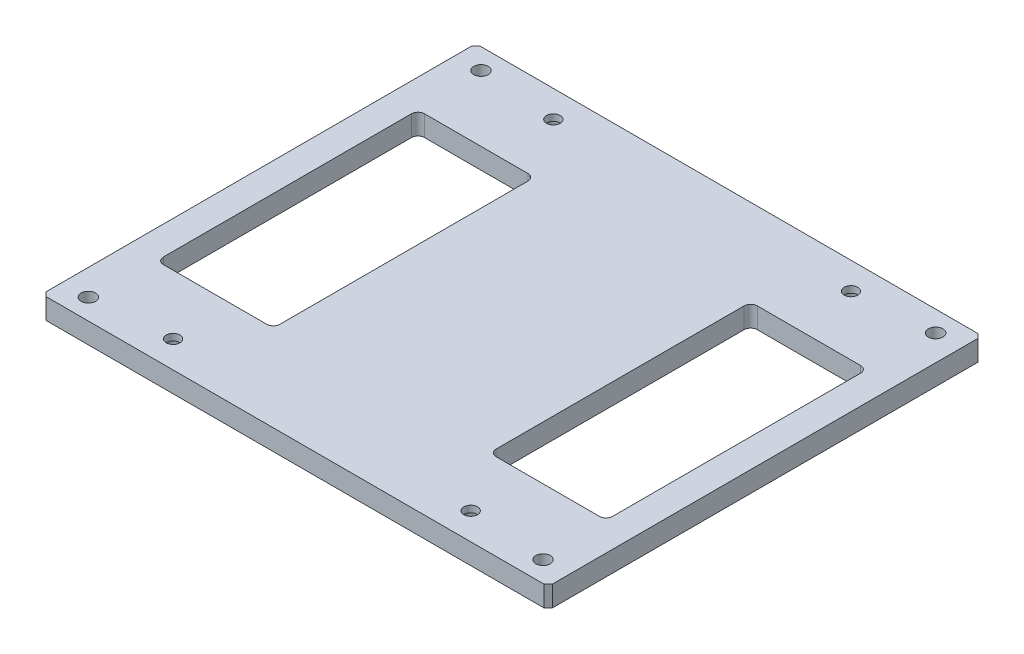
SolidWorks part; units mm, degrees
ref_plane "前视基准面" through (0, 0, 0) normal (0, 0, 1) x (1, 0, 0)
ref_plane "上视基准面" through (0, 0, 0) normal (0, 1, 0) x (1, 0, 0)
ref_plane "右视基准面" through (0, 0, 0) normal (1, 0, 0) x (0, 0, -1)
sketch "草图1" plane through (0, 0, 0) normal (0, 1, 0) x (1, 0, 0)
  line L1 (-122.5, -105) -> (122.5, -105)
  line L2 (-122.5, -105) -> (-122.5, 105)
  line L3 (-122.5, 105) -> (122.5, 105)
  line L4 (122.5, -105) -> (122.5, 105)
  line L5 (-122.5, -105) -> (122.5, 105) construction
  line L6 (-122.5, 105) -> (122.5, -105) construction
  point P0 (0, 0)
  dimension "D1" = 210
  dimension "D2" = 245
extrude "凸台-拉伸1" add sketch "草图1" along normal blind 10
sketch "草图3" plane through (0, 0, 0) normal (0, -1, 0) x (1, 0, 0)
  line L1 (-122.5, 105) -> (122.5, 105) construction
  circle A0 centre (72, 92) radius 3.5
  dimension "D1" = 7
  dimension "D2" = 72
  dimension "D3" = 13
chamfer "倒角1" distance 2 angle 45 4 edges at (-122.5, 5, 105) (-122.5, 5, -105) (122.5, 5, -105) (122.5, 5, 105)
hole_wizard "打孔尺寸(%根据)内六角圆柱头螺钉的类型1" positions "3D草图1" profile "草图4" counterbore size "M6" standard "GB" end condition up to next
sketch3d "3D草图1"
  point P0 (72, 0, 92)
  point P6 (0, 0, 0)
sketch "草图4" plane through (72, 0, 92) normal (1, 0, 0) x (0, 0, -1)
  line L0 (0, 0) -> (0, 10.001)
  line L1 (0, 10.001) -> (3.3, 10.001)
  line L3 (3.3, 10.001) -> (3.3, 6.8)
  line L4 (5.5, 6.8) -> (3.3, 6.8)
  line L5 (5.5, 6.8) -> (5.5, 0.025)
  line L6 (5.5, 0.025) -> (5.525, 0)
  line L7 (5.525, 0) -> (0, 0)
  line L8 (-5.5, 0.025) -> (-5.525, 0) construction
  line L11 (0, -6.35) -> (0, 107.95) construction
  dimension "通孔孔直径" = 6.6
  dimension "通孔孔深度" = 10.001
  dimension "柱形沉头孔直径" = 11
  dimension "柱形沉头孔深度" = 6.8
  dimension "近端锥形沉头孔直径" = 11.05
  dimension "近端锥形沉头孔角度" = 90
mirror "镜向1" about plane through (0, 0, 0) normal (1, 0, 0) of "打孔尺寸(%根据)内六角圆柱头螺钉的类型1"
mirror "镜向2" about plane through (0, 0, 0) normal (0, 0, 1) of "镜向1", "打孔尺寸(%根据)内六角圆柱头螺钉的类型1"
sketch "草图5" plane through (0, 10, 0) normal (0, 1, 0) x (1, 0, 0)
  line L0 (120.5, 105) -> (-120.5, 105) construction
  line L1 (-110, -95) -> (110, -95) construction
  line L2 (-110, -95) -> (-110, 95) construction
  line L3 (-110, 95) -> (110, 95) construction
  line L4 (110, -95) -> (110, 95) construction
  line L5 (-110, -95) -> (110, 95) construction
  line L6 (-110, 95) -> (110, -95) construction
  circle A0 centre (-110, 95) radius 3.5
  circle A1 centre (110, 95) radius 3.5
  circle A2 centre (110, -95) radius 3.5
  circle A3 centre (-110, -95) radius 3.5
  point P0 (0, 0)
  dimension "D3" = 7
  dimension "D1" = 10
  dimension "D2" = 110
extrude "切除-拉伸1" cut sketch "草图5" against normal up to next
sketch "草图6" plane through (0, 10, 0) normal (0, 1, 0) x (1, 0, 0)
  line L0 (105.5, -63.2) -> (55.5, -63.2) construction
  line L1 (108.7, 60) -> (108.7, -60) construction
  line L2 (55.5, 63.2) -> (105.5, 63.2) construction
  line L3 (52.3, -60) -> (52.3, 60) construction
  line L4 (105.5, -63.2) -> (55.5, -63.2)
  line L5 (108.7, 60) -> (108.7, -60)
  line L6 (55.5, 63.2) -> (105.5, 63.2)
  line L7 (52.3, -60) -> (52.3, 60)
  arc A0 (52.3, -60) -> (55.5, -63.2) centre (55.5, -60) ccw construction
  arc A1 (105.5, -63.2) -> (108.7, -60) centre (105.5, -60) ccw construction
  arc A2 (108.7, 60) -> (105.5, 63.2) centre (105.5, 60) ccw construction
  arc A3 (55.5, 63.2) -> (52.3, 60) centre (55.5, 60) ccw construction
  arc A4 (52.3, -60) -> (55.5, -63.2) centre (55.5, -60) ccw
  arc A5 (105.5, -63.2) -> (108.7, -60) centre (105.5, -60) ccw
  arc A6 (108.7, 60) -> (105.5, 63.2) centre (105.5, 60) ccw
  arc A7 (55.5, 63.2) -> (52.3, 60) centre (55.5, 60) ccw
extrude "切除-拉伸2" cut sketch "草图6" against normal up to next
mirror "镜向3" about plane through (0, 0, 0) normal (1, 0, 0) of "切除-拉伸2"
